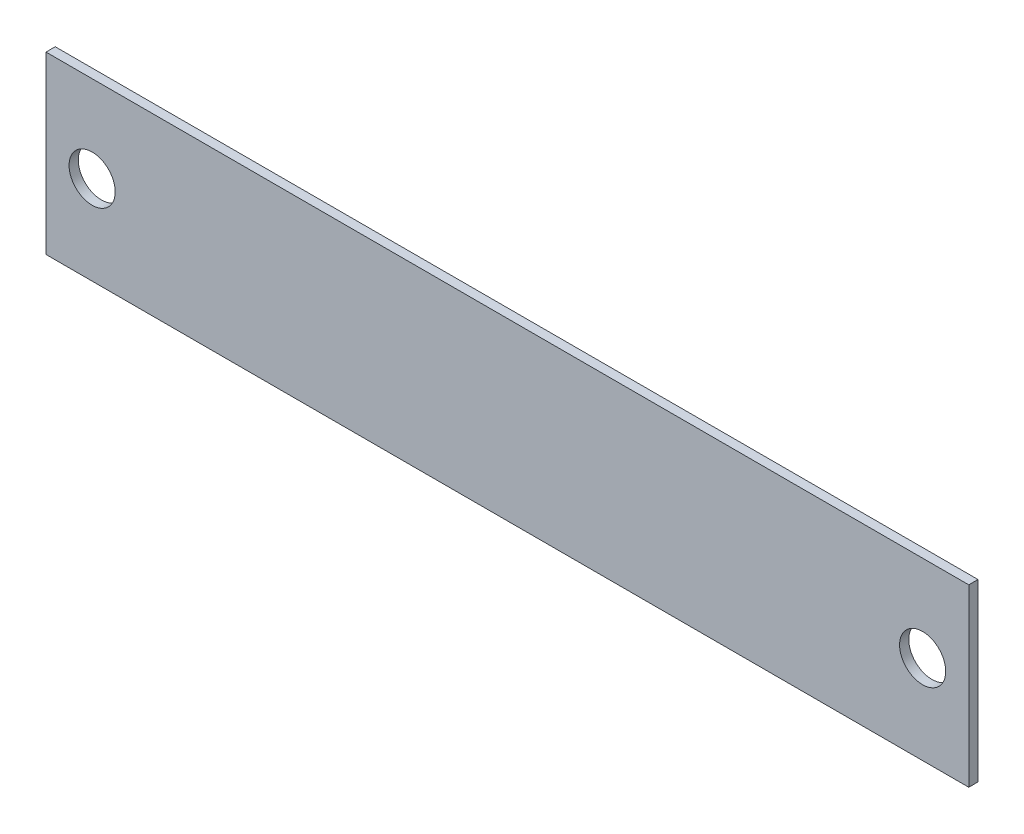
SolidWorks part; units mm, degrees
ref_plane "前视基准面" through (0, 0, 0) normal (0, 0, 1) x (1, 0, 0)
ref_plane "上视基准面" through (0, 0, 0) normal (0, 1, 0) x (1, 0, 0)
ref_plane "右视基准面" through (0, 0, 0) normal (1, 0, 0) x (0, 0, -1)
sketch "草图1" plane through (0, 0, 0) normal (0, 0, 1) x (1, 0, 0)
  line L1 (-50, 19) -> (50, 19)
  line L2 (-50, 19) -> (-50, 0)
  line L3 (-50, 0) -> (50, 0)
  line L4 (50, 19) -> (50, 0)
  dimension "D1" = 100
  dimension "D2" = 19
extrude "凸台-拉伸1" add sketch "草图1" along normal blind 1
hole_wizard "Ø5.0 (5) 直径孔1" positions "草图3" profile "草图2" hole size "Ø5.0" standard "GB" end condition through all
sketch "草图3" plane through (0, 0, 1) normal (0, 0, 1) x (1, 0, 0)
  line L0 (50, 0) -> (50, 19) construction
  line L1 (-50, 19) -> (-50, 0) construction
  point P0 (-45, 9.6219)
  point P2 (45, 9.6219)
  point P7 (-50, 9.5)
  dimension "D1" = 5
  dimension "D2" = 5
sketch "草图2" plane through (-45, 9.6219, 1) normal (1, 0, 0) x (0, -1, 0)
  line L0 (0, 0) -> (0, 1)
  line L1 (0, 1) -> (2.5, 1)
  line L2 (2.5, 1) -> (2.5, 0)
  line L5 (2.5, 0) -> (0, 0)
  line L11 (0, -6.35) -> (0, 107.95) construction
  dimension "通孔孔直径" = 5
  dimension "通孔孔深度" = 1
